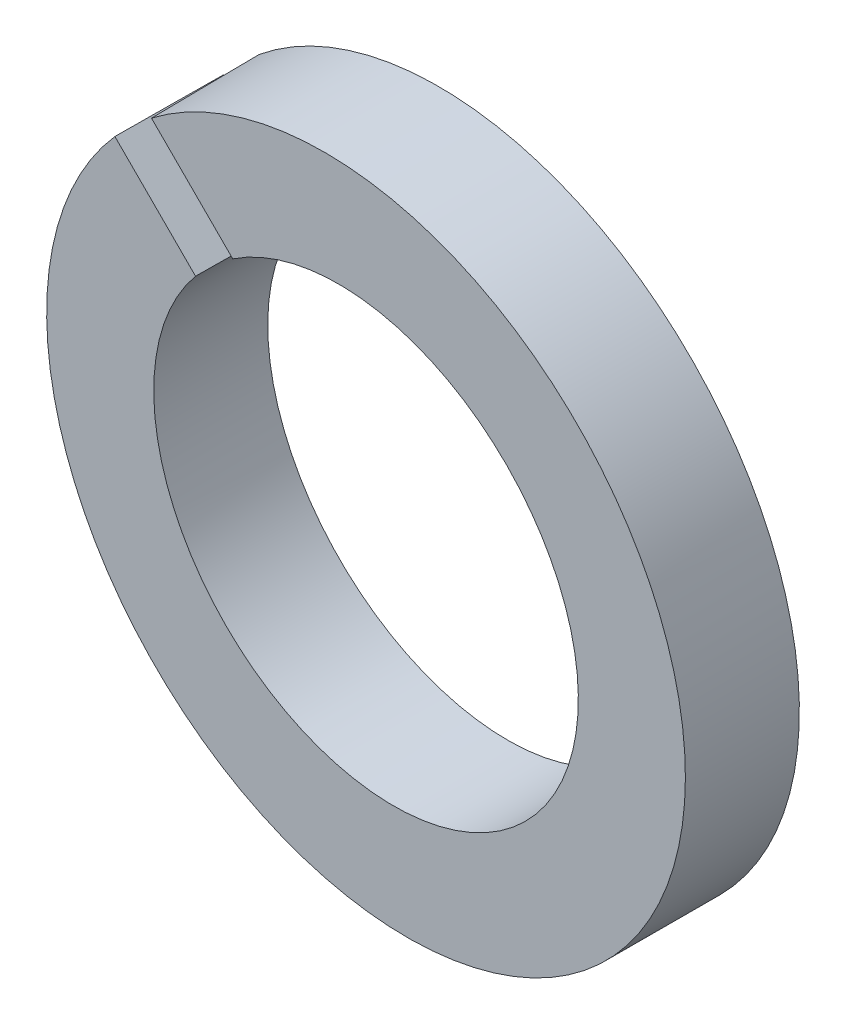
from build123d import *

# Parameters (mm, degrees)
BASE_EXTRUDE_DEPTH      = 0.001
BASE_EXTRUDE_DEPTH_BACK = 0.001
SKETCH6_W               = 6.42
SKETCH6_H               = 6.76
SKETCH8_R               = 20.30887065
SKETCH8_R_2             = 13.5
BOSS_EXTRUDE1_DEPTH     = 6.46
CUT_EXTRUDE1_DEPTH      = 31.552378082
CUT_EXTRUDE1_DEPTH_BACK = 31.552378082


with BuildPart() as part:
    # Sketch6 → Base-Extrude (new, two sides: drawn at the far end of the back side and taken through both)
    with BuildSketch(Plane(origin=(-9.545941546, 9.545941546, 7.14), x_dir=(0.05931115895295759, 0.059311158952956106, -0.996475977054798), z_dir=(0.7046149206649441, 0.7046149206649323, 0.08387864539133799)).offset(-BASE_EXTRUDE_DEPTH_BACK)):
        with Locations((3.23, 3.4)):
            Rectangle(SKETCH6_W, SKETCH6_H)
    extrude(amount=BASE_EXTRUDE_DEPTH + BASE_EXTRUDE_DEPTH_BACK)

    # Sketch8 → Boss-Extrude1 (add)
    with BuildSketch(Plane(origin=(-0.420803093, -0.420803093, 7.069836103), x_dir=(0.9982394983905275, -0.0038244762114057976, 0.05918848903914046), z_dir=(-0.05931115895295754, -0.05931115895295616, 0.996475977054798))):
        with Locations(Location((0, 0, 0), (0, 0, 0.219513325))):
            Circle(SKETCH8_R)
        with Locations(Location((0, 0, 0), (0, 0, 0.219513325))):
            Circle(SKETCH8_R_2, mode=Mode.SUBTRACT)
    extrude(amount=-BOSS_EXTRUDE1_DEPTH)

    # Sketch9 → Cut-Extrude1 (cut, two sides: drawn at the far end of the back side and taken through both)
    with BuildSketch(Plane.XY.offset(-CUT_EXTRUDE1_DEPTH_BACK)):
        Polygon((-34.048869909, 36.453032965), (0.95291576, 1.451247296), (-1.451247296, -0.95291576), (-38.857196021, 36.453032965), align=None)
    extrude(amount=CUT_EXTRUDE1_DEPTH + CUT_EXTRUDE1_DEPTH_BACK, mode=Mode.SUBTRACT)


solid = part.part
